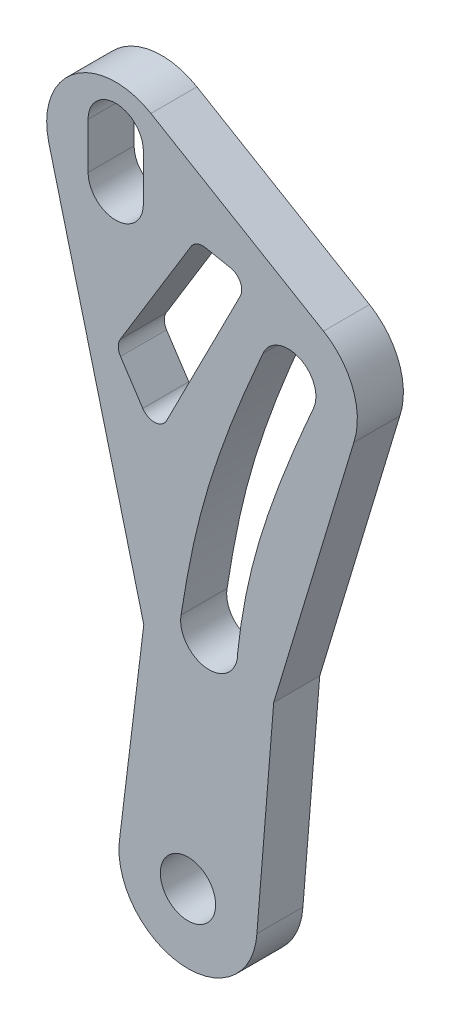
from build123d import *

# Parameters (mm, degrees)
BOSS_EXTRUDE1_DEPTH = 10
CUT_EXTRUDE8_DEPTH  = 10
SKETCH21_R          = 6
CUT_EXTRUDE14_DEPTH = 36
CUT_EXTRUDE15_DEPTH = 10
SKETCH19_R          = 125.517206862
CUT_EXTRUDE16_DEPTH = 10


with BuildPart() as part:
    # Sketch1 → Boss-Extrude1 (new body)
    with BuildSketch(Plane.XY):
        Polygon((0, 0), (0, 170), (100, 170), (100, 0), (100, -20), (0, -20), align=None)
    extrude(amount=BOSS_EXTRUDE1_DEPTH)

    # Sketch9 → Cut-Extrude8 (cut)
    with BuildSketch(Plane.XY.offset(10)):
        with BuildLine():
            Line((29.787758795, 148.908841534), (29.787758795, 138.908841534))
            ThreePointArc((29.787758795, 138.908841534), (35.787758795, 132.908841534), (41.787758795, 138.908841534))
            Line((41.787758795, 138.908841534), (41.787758795, 148.908841534))
            ThreePointArc((41.787758795, 148.908841534), (35.787758795, 154.908841534), (29.787758795, 148.908841534))
        make_face()
    extrude(amount=-CUT_EXTRUDE8_DEPTH, mode=Mode.SUBTRACT)

    # Sketch21 → Cut-Extrude14 (cut)
    with BuildSketch(Plane(origin=(0, 0, 0), x_dir=(-1, 0, 0), z_dir=(0, 0, -1))):
        with Locations((-51.483180233, 14.944928588)):
            Circle(SKETCH21_R)
        with Locations((-173.125589471, 5.899139524)):
            Circle(SKETCH21_R)
    extrude(amount=-CUT_EXTRUDE14_DEPTH, mode=Mode.SUBTRACT)

    # Sketch28 → Cut-Extrude15 (cut)
    with BuildSketch(Plane.XY.offset(10)):
        with BuildLine():
            ThreePointArc((78.796565751, 119.119536449), (75.600421883, 126.979858603), (67.740099728, 123.783714736))
            add(Edge.make_bspline(
                [(67.740099728, 123.783714736), (64.092305086, 115.480107597), (59.109492341, 103.369529902), (53.161827647, 83.940069885), (51.100576539, 72.87588046), (49.983799811, 65.743090583)],
                knots=[0, 0, 0, 0, 0.446952238, 0.644100667, 1, 1, 1, 1], degree=3))
            ThreePointArc((49.983799811, 65.743090583), (55.659355828, 58.49601037), (62.288867459, 64.882064178))
            add(Edge.make_bspline(
                [(78.796565751, 119.119536449), (75.230202559, 110.937069208), (70.252785241, 99.033521906), (65.59137225, 83.75023837), (63.459360665, 73.923916137), (62.602399905, 67.882836475), (62.288867459, 64.882064178)],
                knots=[0, 0, 0, 0, 0.457699653, 0.660132463, 0.817976892, 0.972547387, 0.972547387, 0.972547387, 0.972547387], degree=3))
        make_face()
    extrude(amount=-CUT_EXTRUDE15_DEPTH, mode=Mode.SUBTRACT)

    # Sketch19 → Cut-Extrude16 (cut)
    # profile 1 of 2: a face of its own
    with BuildSketch(Plane.XY.offset(10)):
        with Locations((58.773015823, 71.241859079)):
            Circle(SKETCH19_R)
        with BuildLine():
            Line((41.881776011, 59.878203095), (36.689834848, 17.426245238))
            ThreePointArc((36.689834848, 17.426245238), (49.776196121, 0.042371585), (66.454445821, 14.016916355))
            Line((66.454445821, 14.016916355), (70.10422157, 59.327257721))
            Line((70.10422157, 59.327257721), (70.725023214, 61.382630275))
            Line((70.725023214, 61.382630275), (87.508098537, 116.948643541))
            ThreePointArc((87.508098537, 116.948643541), (87.335113551, 126.939388183), (80.925197211, 134.604756721))
            Line((80.925197211, 134.604756721), (43.432736819, 156.814433772))
            ThreePointArc((43.432736819, 156.814433772), (26.883190667, 155.979826019), (21.200543901, 140.414108121))
            Line((21.200543901, 140.414108121), (41.325983429, 62.042545062))
            Line((41.325983429, 62.042545062), (41.881776011, 59.878203095))
        make_face(mode=Mode.SUBTRACT)
    # profile 2 of 2: a face of its own
    with BuildSketch(Plane.XY.offset(10)):
        with BuildLine():
            Line((52.121181326, 136.108026927), (36.779697673, 111.015745375))
            ThreePointArc((36.779697673, 111.015745375), (36.33960448, 109.402281892), (36.831704565, 107.803912744))
            Line((36.831704565, 107.803912744), (41.662593186, 100.448764157))
            ThreePointArc((41.662593186, 100.448764157), (44.33499195, 99.10023877), (46.84322719, 100.733943719))
            Line((46.84322719, 100.733943719), (62.827881658, 132.111730058))
            ThreePointArc((62.827881658, 132.111730058), (62.851731636, 134.787382647), (60.730080577, 136.417806633))
            Line((60.730080577, 136.417806633), (55.25602114, 137.487450431))
            ThreePointArc((55.25602114, 137.487450431), (53.472410109, 137.289048664), (52.121181326, 136.108026927))
        make_face()
    extrude(amount=-CUT_EXTRUDE16_DEPTH, mode=Mode.SUBTRACT)


solid = part.part
